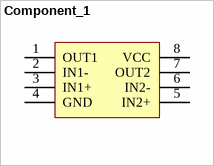
[diagram p0: symbol Component_1]
# Altium schematic symbol library MISC86340-20.SchLib: 1 symbol
Pins are listed as number, name and electrical type; pins without a type are passive.


## Component_1
designator ?
footprint LM393
pins: 1 OUT1, 2 IN1-, 3 IN1+, 4 GND, 5 IN2+, 6 IN2-, 7 OUT2, 8 VCC